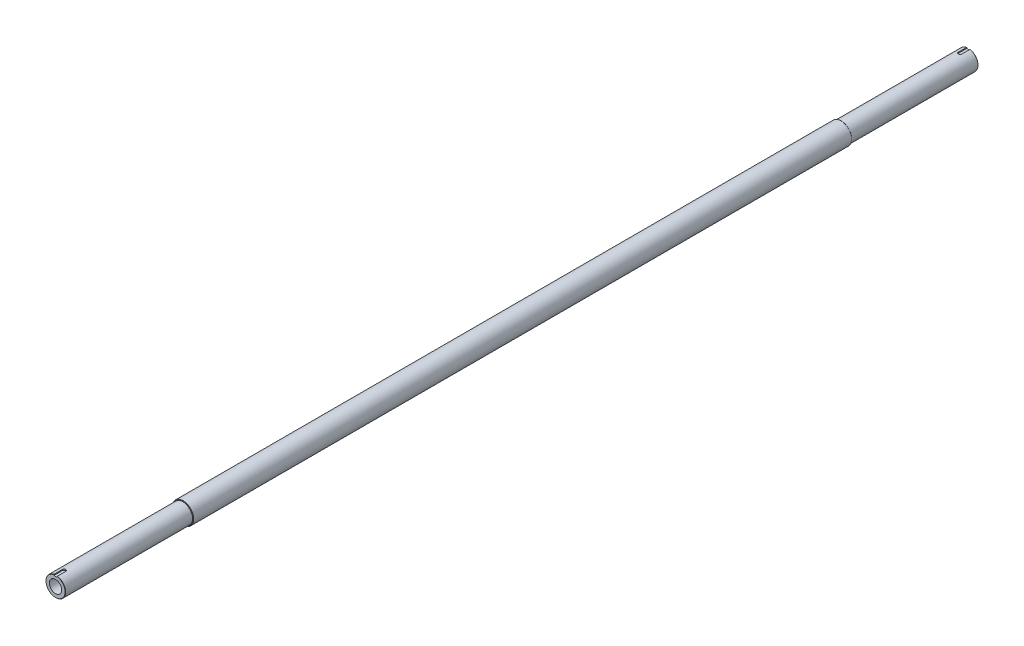
from build123d import *

# Parameters (mm, degrees)
SKETCH1_R           = 38
BOSS_EXTRUDE1_DEPTH = 3254
SKETCH2_R           = 38
SKETCH2_R_2         = 35
CUT_EXTRUDE1_DEPTH  = 453.5
CUT_EXTRUDE2_START  = -453.5
SKETCH3_R           = 38
SKETCH3_R_2         = 35
CUT_EXTRUDE2_DEPTH  = 453.5
SKETCH5_R           = 22
CUT_EXTRUDE3_DEPTH  = 3255.44373127
CUT_EXTRUDE4_DEPTH  = 4
CHAMFER1_SIZE       = 1


with BuildPart() as part:
    # Sketch1 → Boss-Extrude1 (new body)
    with BuildSketch(Plane.XY):
        Circle(SKETCH1_R)
    extrude(amount=BOSS_EXTRUDE1_DEPTH)

    # Sketch2 → Cut-Extrude1 (cut)
    with BuildSketch(Plane(origin=(0, 0, 0), x_dir=(-1, 0, 0), z_dir=(0, 0, -1))):
        Circle(SKETCH2_R)
        Circle(SKETCH2_R_2, mode=Mode.SUBTRACT)
    extrude(amount=-CUT_EXTRUDE1_DEPTH, mode=Mode.SUBTRACT)

    # Sketch3 → Cut-Extrude2 (cut)
    with BuildSketch(Plane.XY.offset(3254).offset(CUT_EXTRUDE2_START)):
        with Locations(Location((0, 0, 0), (0, 0, 180))):
            Circle(SKETCH3_R)
        with Locations(Location((0, 0, 0), (0, 0, 180))):
            Circle(SKETCH3_R_2, mode=Mode.SUBTRACT)
    extrude(amount=CUT_EXTRUDE2_DEPTH, mode=Mode.SUBTRACT)

    # Sketch5 → Cut-Extrude3 (cut, through all)
    with BuildSketch(Plane(origin=(0, 0, 0), x_dir=(-1, 0, 0), z_dir=(0, 0, -1))):
        Circle(SKETCH5_R)
    extrude(amount=-CUT_EXTRUDE3_DEPTH, mode=Mode.SUBTRACT)

    # Sketch6 → Cut-Extrude4 (cut)
    with BuildSketch(Plane(origin=(0, 35, 0), x_dir=(1, 0, 0), z_dir=(0, 1, 0))):
        with BuildLine():
            Line((6, 0), (6, -30))
            ThreePointArc((6, -30), (0, -36), (-6, -30))
            Line((-6, -30), (-6, 0))
            ThreePointArc((-6, 0), (0, 6), (6, 0))
        make_face()
    cut_extrude4 = extrude(amount=-CUT_EXTRUDE4_DEPTH, mode=Mode.SUBTRACT)

    # Mirror1: Cut-Extrude4 across plane
    add(cut_extrude4.mirror(Plane(origin=(0, 0, 1627), x_dir=(1, 0, 0), z_dir=(0, 0, -1))), mode=Mode.SUBTRACT)

    # Chamfer1
    chamfer1_edges = [part.edges().sort_by_distance(p)[0] for p in [
        (-38, 0, 2800.5),
        (22.527760652, -26.786190472, 0),
        (22.527760652, -26.786190472, 3254),
        (-38, 0, 453.5),
    ]]
    chamfer(chamfer1_edges, length=CHAMFER1_SIZE)


solid = part.part
